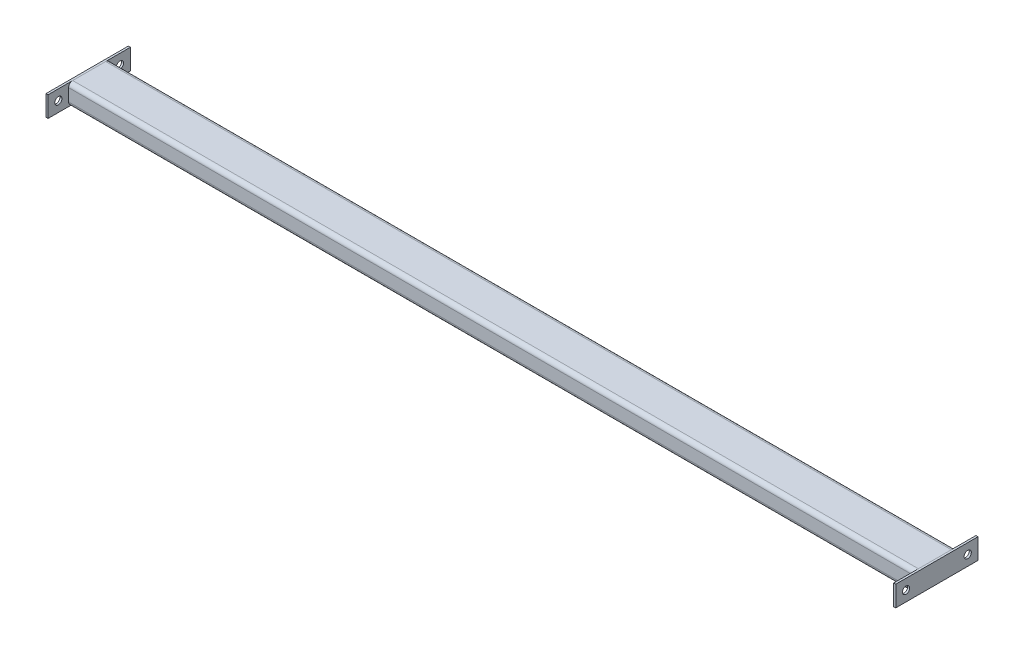
from build123d import *

# Parameters (mm, degrees)
MEMBER_1_DEPTH  = 1234
SKETCH_3_W      = 120
SKETCH_3_H      = 30
SKETCH_3_R      = 5.25
EXTRUDE_1_DEPTH = 3


with BuildPart() as part:
    # Sketch1 → Member 1 (new body)
    with BuildSketch(Plane.YZ.offset(-617)):
        with BuildLine():
            Line((-9, -30), (9, -30))
            ThreePointArc((9, -30), (13.242640687, -28.242640687), (15, -24))
            Line((15, -24), (15, 24))
            ThreePointArc((15, 24), (13.242640687, 28.242640687), (9, 30))
            Line((9, 30), (-9, 30))
            ThreePointArc((-9, 30), (-13.242640687, 28.242640687), (-15, 24))
            Line((-15, 24), (-15, -24))
            ThreePointArc((-15, -24), (-13.242640687, -28.242640687), (-9, -30))
        make_face()
        with BuildLine():
            Line((-9, -27), (9, -27))
            ThreePointArc((9, -27), (11.121320344, -26.121320344), (12, -24))
            Line((12, -24), (12, 24))
            ThreePointArc((12, 24), (11.121320344, 26.121320344), (9, 27))
            Line((9, 27), (-9, 27))
            ThreePointArc((-9, 27), (-11.121320344, 26.121320344), (-12, 24))
            Line((-12, 24), (-12, -24))
            ThreePointArc((-12, -24), (-11.121320344, -26.121320344), (-9, -27))
        make_face(mode=Mode.SUBTRACT)
    extrude(amount=MEMBER_1_DEPTH)


with BuildPart() as body_2:
    # 草图3 → 凸台-拉伸1 (new body)
    with BuildSketch(Plane(origin=(617, 0, 0), x_dir=(0, 0, -1), z_dir=(1, 0, 0))):
        Rectangle(SKETCH_3_W, SKETCH_3_H)
        with Locations((45, 0)):
            Circle(SKETCH_3_R, mode=Mode.SUBTRACT)
        with Locations(Location((-45, 0, 0), (0, 0, 180))):
            Circle(SKETCH_3_R, mode=Mode.SUBTRACT)
    extrude(amount=EXTRUDE_1_DEPTH)


with BuildPart() as body_3:
    # 镜向1: mirrored copy
    add(body_2.part.mirror(Plane(origin=(0, 0, 0), x_dir=(0, 0, 1), z_dir=(1, 0, 0))))


solid = Compound([part.part, body_2.part, body_3.part])
